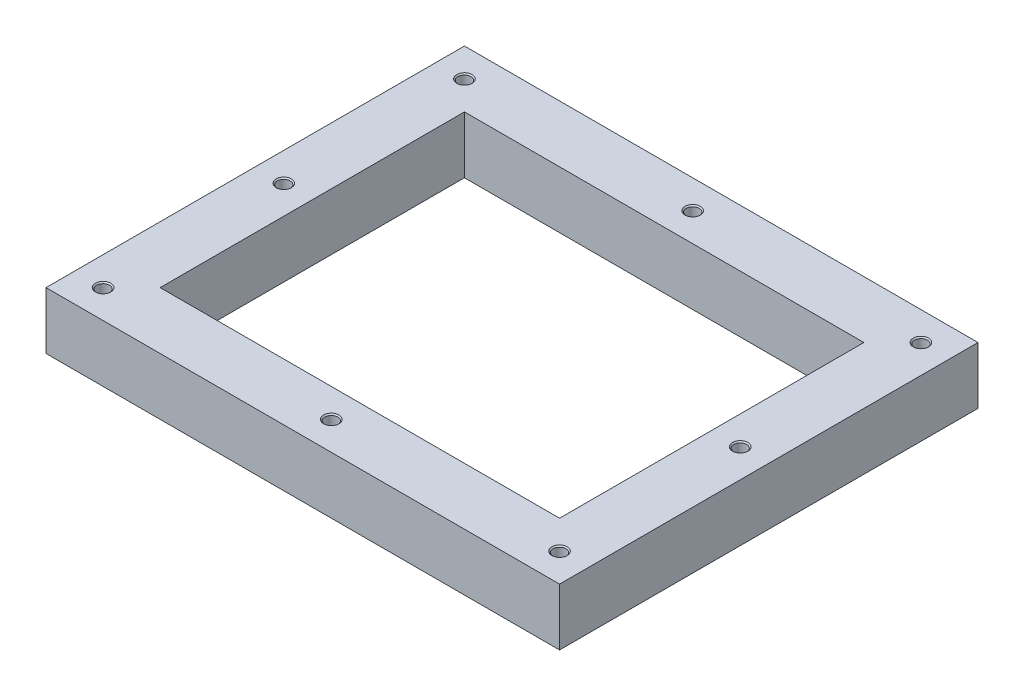
SolidWorks part; units mm, degrees
ref_plane "Front Plane" through (0, 0, 0) normal (0, 0, 1) x (1, 0, 0)
ref_plane "Top Plane" through (0, 0, 0) normal (0, 1, 0) x (1, 0, 0)
ref_plane "Right Plane" through (0, 0, 0) normal (1, 0, 0) x (0, 0, -1)
sketch "Sketch1" plane through (0, 0, 0) normal (0, 1, 0) x (1, 0, 0)
  line L1 (-135, 110) -> (135, 110)
  line L2 (-135, 110) -> (-135, -110)
  line L3 (-135, -110) -> (135, -110)
  line L4 (135, 110) -> (135, -110)
  line L5 (-135, 110) -> (135, -110) construction
  line L6 (-135, -110) -> (135, 110) construction
  line L7 (-105, 80) -> (105, 80)
  line L8 (-105, 80) -> (-105, -80)
  line L9 (-105, -80) -> (105, -80)
  line L10 (105, 80) -> (105, -80)
  line L11 (-105, 80) -> (105, -80) construction
  line L12 (-105, -80) -> (105, 80) construction
  point P0 (0, 0)
  point P6 (0, 0)
  dimension "D1" = 270
  dimension "D2" = 220
  dimension "D3" = 210
  dimension "D4" = 160
extrude "Boss-Extrude1" add sketch "Sketch1" along normal blind 30
hole_wizard "M8 Tapped Hole1" positions "Sketch5" profile "Sketch6" tap size "M8" standard "GB"
sketch "Sketch5" plane through (0, 30, 0) normal (0, 1, 0) x (1, 0, 0)
  line L0 (0, 123.7558) -> (0, -143.0571) construction
  line L2 (-135, 110) -> (-135, -110) construction
  line L3 (-120, 95) -> (-120, -137.2497) construction
  line L5 (-135, -110) -> (135, -110) construction
  line L6 (-120, 95) -> (135, 95) construction
  line L7 (135, -110) -> (135, 110) construction
  line L10 (120, 95) -> (120, -137.2497) construction
  point P0 (0, 95)
  point P2 (-120, 95)
  point P4 (-120, 0)
  point P6 (-120, -95)
  point P8 (0, -95)
  point P36 (120, -95)
  point P39 (120, 95)
  point P41 (120, 0)
  dimension "D1" = 120
  dimension "D2" = 15
  dimension "D3" = 95
  dimension "D4" = 95
  dimension "D5" = 15
  dimension "D6" = 15
sketch "Sketch6" plane through (0, 30, -95) normal (1, 0, 0) x (0, 0, 1)
  line L0 (0, 0) -> (0, 23.75)
  line L1 (0, 23.75) -> (3.4, 21.7071)
  line L2 (3.4, 21.7071) -> (3.4, 0.625)
  line L3 (3.4, 0.625) -> (4.025, 0)
  line L5 (4.025, 0) -> (0, 0)
  line L6 (-3.4, 0.625) -> (-4.025, 0) construction
  line L10 (0, 23.75) -> (-3.4, 21.7071) construction
  line L11 (0, -6.35) -> (0, 107.95) construction
  dimension "螺纹孔钻头直径" = 6.8
  dimension "螺纹孔钻头深度" = 23.75
  dimension "近端锥形沉头孔直径" = 8.05
  dimension "近端锥形沉头孔角度" = 90
  dimension "导头角度" = 118
cosmetic thread "Cosmetic thread 1" parameters "D1"=20, "D2"=8
cosmetic thread "Cosmetic thread 2" parameters "D1"=20, "D2"=8
cosmetic thread "Cosmetic thread 3" parameters "D1"=20, "D2"=8
cosmetic thread "Cosmetic thread 4" parameters "D1"=20, "D2"=8
cosmetic thread "Cosmetic thread 5" parameters "D1"=20, "D2"=8
cosmetic thread "Cosmetic thread 6" parameters "D1"=20, "D2"=8
cosmetic thread "Cosmetic thread 7" parameters "D1"=20, "D2"=8
cosmetic thread "Cosmetic thread 8" parameters "D1"=20, "D2"=8
